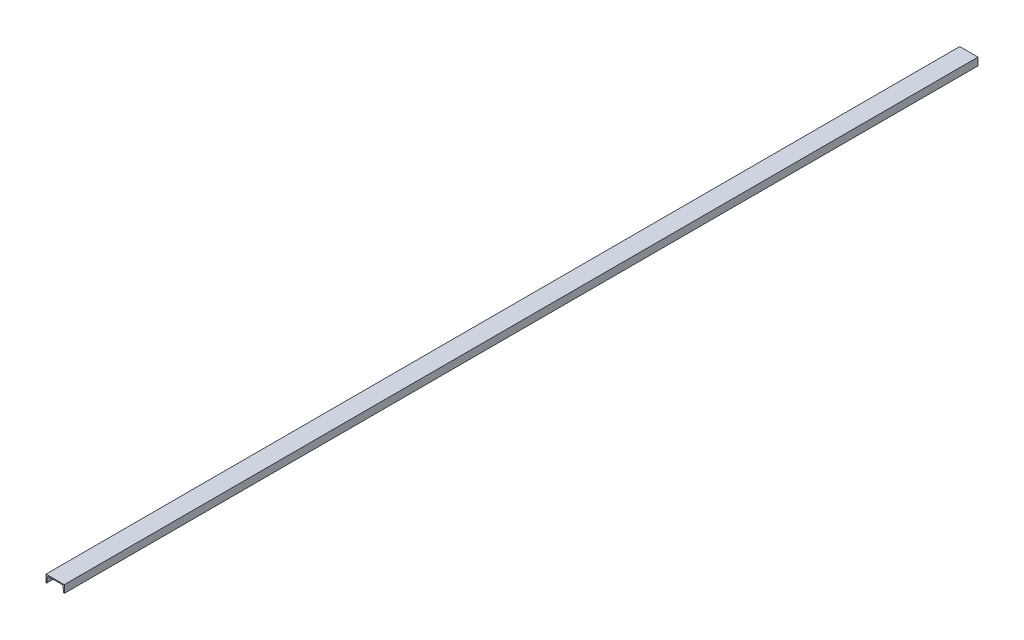
SolidWorks part; units mm, degrees
material "普通碳钢"
ref_plane "Front Plane" through (0, 0, 0) normal (0, 0, 1) x (1, 0, 0)
ref_plane "Top Plane" through (0, 0, 0) normal (0, 1, 0) x (1, 0, 0)
ref_plane "Right Plane" through (0, 0, 0) normal (1, 0, 0) x (0, 0, -1)
sketch "Sketch1" plane through (0, 0, 0) normal (0, 0, 1) x (1, 0, 0)
  line L0 (0, 0) -> (0, 50)
  line L1 (0, 50) -> (120, 50)
  line L2 (120, 50) -> (120, 0)
  line L3 (0, 0) -> (2.5485, 0)
  line L4 (4.5356, 1.7732) -> (8.7527, 38.7239)
  line L5 (13.7205, 43.1569) -> (106.2795, 43.1569)
  line L6 (60, 50) -> (60, 36.5447) construction
  line L7 (120, 0) -> (117.4515, 0)
  line L8 (115.4644, 1.7732) -> (111.2473, 38.7239)
  arc A0 (8.7527, 38.7239) -> (13.7205, 43.1569) centre (13.7205, 38.1569) cw
  arc A1 (4.5356, 1.7732) -> (2.5485, 0) centre (2.5485, 2) cw
  arc A2 (111.2473, 38.7239) -> (106.2795, 43.1569) centre (106.2795, 38.1569) ccw
  arc A3 (115.4644, 1.7732) -> (117.4515, 0) centre (117.4515, 2) ccw
  point P15 (60, 43.1569)
  dimension "D4" = 5
  dimension "D5" = 2
  dimension "D1" = 120
  dimension "D3" = 50
extrude "Boss-Extrude1" add sketch "Sketch1" along normal blind 6000
